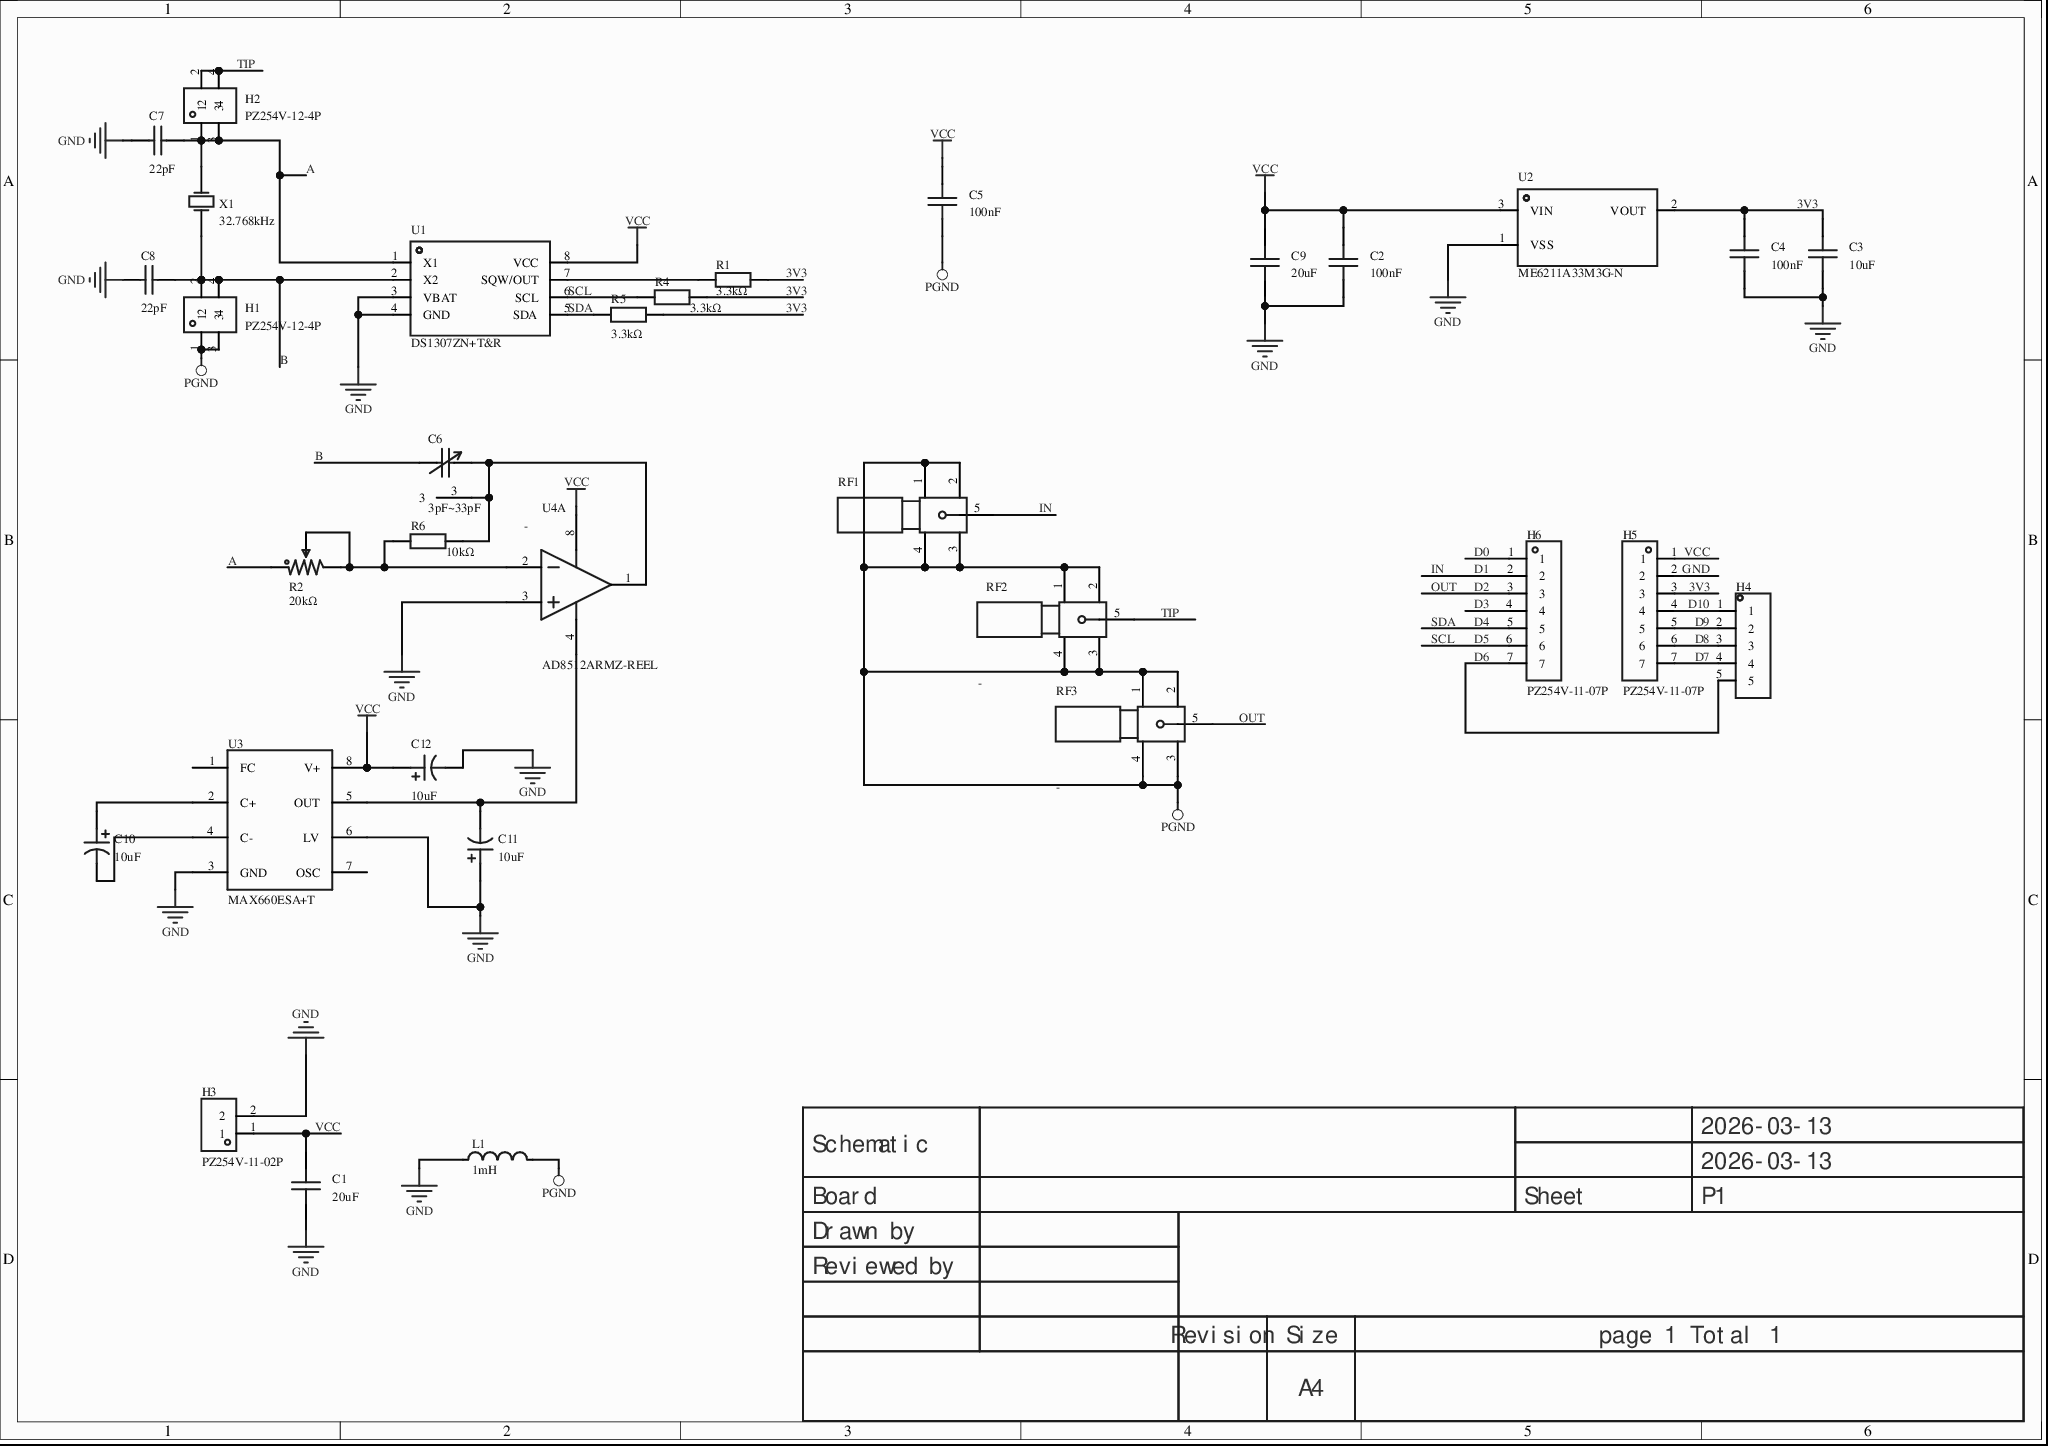
[diagram p0: MISC75269-3.schdoc]
# Altium project MISC75269-2.PrjPcb
1 sheet, 32 parts. Net scope: global (net labels, ports and power ports of the same name join across sheets).
Board file: MISC75269.pcbdoc

## Sheet MISC75269-3.schdoc
size 297 x 209 mm; Version: V1.0; @Project Name: MISC75269; @Update Date: 2026-03-13; @Create Date: 2026-03-13; @Board Name: MISC75269; @Create Time: 17:50:26; @Page Count: 1; @Page No: 1; @Schematic Name: MISC75269; @Update Time: 17:50:26; Size: A4

### Parts
C1  20uF  [CAP-SMD_L1.8-W1.0]
C2  100nF  [C0603]
C3  10uF  [C0603]
C4  100nF  [C0603]
C5  100nF  [C0603]
C6  3pF~33pF  [CAP-ADJ-TH_3P-BD7.6_BFC280811339]
C7  22pF  [C0603]
C8  22pF  [C0603]
C9  20uF  [CAP-SMD_L1.8-W1.0]
C10  10uF  [CAP-SMD_BD5.0-L5.3-W5.3-LS6.0-FD]
C11  10uF  [CAP-SMD_BD5.0-L5.3-W5.3-LS6.0-FD]
C12  10uF  [CAP-SMD_BD5.0-L5.3-W5.3-LS6.0-FD]
H1  PZ254V-12-4P  [HDR-TH_4P-P2.54-V-M-R2-C2-S2.54]
H2  PZ254V-12-4P  [HDR-TH_4P-P2.54-V-M-R2-C2-S2.54]
H3  PZ254V-11-02P  [HDR-TH_2P-P2.54-V-M]
H4  (no value)  [HDR-TH_5P-P2.54-V-M]
H5  PZ254V-11-07P  [HDR-TH_7P-P2.54-V-M]
H6  PZ254V-11-07P  [HDR-TH_7P-P2.54-V-M]
L1  1mH  [IND-TH_BD8.5-P5.00-D0.6]
R1  3.3kΩ  [R0603]
R2  20kΩ  [RES-ADJ-TH_3362P]
R4  3.3kΩ  [R0603]
R5  3.3kΩ  [R0603]
R6  10kΩ  [R0603]
RF1  -  [SMA-TH_KH-SMA-KE-Z]
RF2  -  [SMA-TH_KH-SMA-KE-Z]
RF3  -  [SMA-TH_KH-SMA-KE-Z]
U1  DS1307ZN+T&R  [SOP-8_L4.9-W3.9-P1.27-LS6.0-BL]
U2  ME6211A33M3G-N  [SOT-23-3_L2.9-W1.6-P1.90-LS2.8-BR]
U3  MAX660ESA+T  [SOIC-8_L5.0-W4.0-P1.27-LS6.0-BL]
U4  AD8512ARMZ-REEL  [MSOP-8_L3.0-W3.0-P0.65-LS5.0-TL]  (part A of 2)
X1  32.768kHz  [OSC-TH_BD3.1-P0.8-D0.3]

### Nets
GND: C1.1 C2.1 C3.1 C4.1 C7.2 C8.2 C9.1 C11.1 C12.2 H3.2 H5.2 L1.1 U1.3(VBAT) U1.4(GND) U2.1(VSS) U3.3(GND) U3.6(LV) U4.3(+IN_A)
PGND: C5.1 H1.1 H1.3 L1.2 RF1.1 RF1.2 RF1.3 RF1.4 RF2.1 RF2.2 RF2.3 RF2.4 RF3.1 RF3.2 RF3.3 RF3.4
VCC: C1.2 C2.2 C5.2 C9.2 C12.1 H3.1 H5.1 U1.8(VCC) U2.3(VIN) U3.8(V+) U4.8(V+)
3V3: C3.2 C4.2 H5.3 R1.2 R4.1 R5.1 U2.2(VOUT)
A: C7.1 H2.1 H2.3 R2.1 U1.1(X1) X1.2(OSC2)
B: C6.1 C8.1 H1.2 H1.4 U1.2(X2) X1.1(OSC1)
D0: H6.1
D1: H6.2 RF1.5  [also labelled IN]
D2: H6.3 RF3.5  [also labelled OUT]
D3: H6.4
D4: H6.5 R5.2 U1.5(SDA)  [also labelled SDA]
D5: H6.6 R4.2 U1.6(SCL)  [also labelled SCL]
D6: H4.5 H6.7
D7: H4.4 H5.7
D8: H4.3 H5.6
D9: H4.2 H5.5
D10: H4.1 H5.4
TIP: H2.2 H2.4 RF2.5
NetC6_2: C6.2 C6.3 R6.1 U4.1(OUT_A)
NetC10_1: C10.1 U3.2(C+)
NetC10_2: C10.2 U3.4(C-)
NetC11_2: C11.2 U3.5(OUT) U4.4(V-)
NetR1_1: R1.1 U1.7(SQW/OUT)
NetR2_2: R2.2 R2.3 R6.2 U4.2(-IN_A)

Not connected (* = marked no-connect by the designer): U3 1(FC)* 7(OSC)*

### Notes on the sheet
- 2026-03-13
- Schematic
- Board
- Sheet
- P1
- Drawn by
- Reviewed by
- Revision
- Size
- A4
- page 1 Total 1

### Library data of the parts
C1 C9 = GRMJN7R61C206ME05D: Capacitance:20uF;Tolerance:±20%;Rated voltage:16V;Temperature coefficient:X5R;; Manufacturer: muRata(村田); AddInBom: yes; ModelId: 7fafba264af843cd9b63e401151876ee0819f05c4eef4c71ace90d822a990e87; ModelTransform: 70.866,39.37394,0,0,0,0,0,0,0; Tolerance: ±20%; Voltage Rating: 16V; Temperature Coefficient: X5R; Symbol: GRMJN7R61C206ME05D; Device: GRMJN7R61C206ME05D; LCSC Part Name: 20uF ±20% 16V; SupplierPart: C6565591; ManufacturerPart: GRMJN7R61C206ME05D; Supplier Footprint: 0704; JLCPCB Part Class: Extended Part; Datasheet: example.com/datasheet/GRMJN7R61C206ME05D/7519706.html; Supplier: LCSC; ConvertToPcb: yes; FootprintName: CAP-SMD_L1.8-W1.0; ModelName: CAP-SMD_L1.8-W1.0; Value: 20uF
C2 C4 C5 = CGA0603X7R104K500JT: Capacitance:100nF;Tolerance:±10%;Rated voltage:50V;Temperature coefficient:X7R;; Manufacturer: HRE(芯声); AddInBom: yes; ModelId: ac125912035d415993ca9572d50418b10819f05c4eef4c71ace90d822a990e87; ModelName: C0603_L1.6-W0.8-H0.8; ModelTransform: 62.992,31.496,0,0,0,0,0,0,0; Tolerance: ±10%; Voltage Rating: 50V; Temperature Coefficient: X7R; Symbol: CGA0603X7R104K500JT; Device: CGA0603X7R104K500JT; LCSC Part Name: 100nF ±10% 50V; SupplierPart: C6119867; ManufacturerPart: CGA0603X7R104K500JT; Supplier Footprint: 0603; JLCPCB Part Class: Extended Part; Datasheet: example.com/datasheet/CGA0603X7R104K500JT/7062573.html; Supplier: LCSC; ConvertToPcb: yes; FootprintName: C0603; Value: 100nF
C3 = CGA0603X5R106K100JT: Capacitance:10uF;Tolerance:±10%;Rated voltage:10V;Temperature coefficient:X5R;; Manufacturer: HRE(芯声); AddInBom: yes; ModelId: ac125912035d415993ca9572d50418b10819f05c4eef4c71ace90d822a990e87; ModelName: C0603_L1.6-W0.8-H0.8; ModelTransform: 62.992,31.496,0,0,0,0,0,0,0; Tolerance: ±10%; Voltage Rating: 10V; Temperature Coefficient: X5R; Symbol: CGA0603X5R106K100JT; Device: CGA0603X5R106K100JT; LCSC Part Name: 10uF ±10% 10V; SupplierPart: C6119842; ManufacturerPart: CGA0603X5R106K100JT; Supplier Footprint: 0603; JLCPCB Part Class: Extended Part; Datasheet: example.com/datasheet/CGA0603X5R106K100JT/7062548.html; Supplier: LCSC; ConvertToPcb: yes; FootprintName: C0603; Value: 10uF
C6 = BFC280811339: Capacitance:3pF~33pF;Rated voltage:250V;Charge:-;; Manufacturer: VISHAY(威世); AddInBom: yes; ModelId: cf28104b1ba149229588c665311718d80819f05c4eef4c71ace90d822a990e87; ModelTransform: 334.645,298.957,0,0,0,0,-15.748,0,-157.48; Voltage Rating: 250V; Symbol: BFC280811339; Device: BFC280811339; LCSC Part Name: 3pF~33pF 250V; SupplierPart: C3273212; ManufacturerPart: BFC280811339; Supplier Footprint: 插件; JLCPCB Part Class: Extended Part; Datasheet: example.com/datasheet/BFC280811339/3836109.html; Supplier: LCSC; ConvertToPcb: yes; FootprintName: CAP-ADJ-TH_3P-BD7.6_BFC280811339; ModelName: CAP-ADJ-TH_3P-BD7.6_BFC280811339; Value: 3pF~33pF; Q @ Frequency: -; Operating Temperature: -40℃~+70℃; Height - Seated(Max): 10mm
C7 C8 = CL10C220JB8NNNC: Capacitance:22pF;Tolerance:±5%;Rated voltage:50V;Temperature coefficient:C0G;; Manufacturer: SAMSUNG(三星); AddInBom: yes; ModelId: ac125912035d415993ca9572d50418b10819f05c4eef4c71ace90d822a990e87; ModelName: C0603_L1.6-W0.8-H0.8; ModelTransform: 62.992,31.496,0,0,0,0,0,0,0; Tolerance: ±5%; Voltage Rating: 50V; Temperature Coefficient: C0G; Symbol: CL10C220JB8NNNC; Device: CL10C220JB8NNNC; LCSC Part Name: 22pF ±5% 50V; SupplierPart: C1653; ManufacturerPart: CL10C220JB8NNNC; Supplier Footprint: 0603; JLCPCB Part Class: Basic Part; Datasheet: example.com/datasheet/CL10C220JB8NNNC/2005.html; Supplier: LCSC; ConvertToPcb: yes; FootprintName: C0603; Value: 22pF
C10-C12 = JVJ50v10M5x5: Capacitance:10uF;Tolerance:±20%;Rated voltage:50V;Ripple current:18mA@120Hz;; Manufacturer: JIERR(捷而瑞); 3D Model: ed942b427de741e3aabba01c64b2d7230819f05c4eef4c71ace90d822a990e87; 3D Model Transform: 236.22,208.661,0,0,0,0,-0.001,-0.003,0; Tolerance: ±20%; Voltage Rating: 50V; Lifetime: 2000hrs@105℃; AddInBom: yes; Symbol: JVJ50V10M5X5; Device: JVJ50v10M5x5; LCSC Part Name: 10uF ±20% 50V; Supplier Part: C46550416; Manufacturer Part: JVJ50v10M5x5; Supplier Footprint: SMD,D5xL5.4mm; JLCPCB Part Class: Extended Part; Datasheet: example.com/datasheet/JVJ50v10M5x5/48680110.html; Supplier: LCSC; Value: 10uF; Ripple Current: 18mA@120Hz; Diameter: 5mm; Height - Seated (Max): 5.4mm; Operating Temperature: -55℃~+105℃; ConvertToPcb: yes; FootprintName: CAP-SMD_BD5.0-L5.3-W5.3-LS6.0-FD; ModelName: CAP-SMD_BD5.0-L5.3-W5.3-LS6.0-FD
H1 H2 = PZ254V-12-4P: Pin structure:2x2P;Pitch:2.54mm;Row spacing:2.54mm;Round/square pin:Square pin;Mounting:Through-hole;Rows:Double row;Total pins:4P;Rated current:-;Rated voltage:-;Mating pin length:6mm;Plastic height:2.5mm;Tail length:3mm;Contact material:Brass;Contact plating:-;Operating temperature:-40℃~+105℃;Color:Black;; Manufacturer: XFCN(兴飞); AddInBom: yes; ModelId: 396726ecc332483f84428c142640bc150819f05c4eef4c71ace90d822a990e87; ModelName: HDR-TH_4P-P2.54-M-LI-2X2P; ModelTransform: 200,200,0,0,0,0,0,0,-118.11; Pin Structure: 2x2P; Pitch: 2.54mm; Circluar Pins/Square Pins: Square; Symbol: PZ254V-12-4P; Device: PZ254V-12-4P; LCSC Part Name: 2x2P 间距:2.54mm 方针 直插; SupplierPart: C492419; ManufacturerPart: PZ254V-12-4P; Supplier Footprint: 插件,P=2.54mm; JLCPCB Part Class: Extended Part; Datasheet: example.com/datasheet/PZ254V-12-4P/502975.html; Supplier: LCSC; ConvertToPcb: yes; FootprintName: HDR-TH_4P-P2.54-V-M-R2-C2-S2.54; Row Spacing: 2.54mm; Mounting Type: Through-hole; Number of Rows: Double row; Number of Pins: 4P; Current Rating: -; Voltage Rating (Max): -; Length of Mating Pin: 6mm; Insulation Height: 2.5mm; Length of End Connection Pin: 3mm; Contact Material: Brass; Contact Plating: -; Operating Temperature: -40℃~+105℃; Color: Black
H3 = PZ254V-11-02P: Pin structure:1x2P;Pitch:2.54mm;Row spacing:-;Round/square pin:Square pin;Mounting:Through-hole;Rows:Single row;Total pins:2P;Rated current:-;Rated voltage:-;Mating pin length:6mm;Plastic height:2.5mm;Tail length:3mm;Contact material:Brass;Contact plating:-;Operating temperature:-40℃~+105℃;Color:Black;; Manufacturer: XFCN(兴飞); AddInBom: yes; ModelId: e35305ec3aa84b66b849f914b715e73f0819f05c4eef4c71ace90d822a990e87; ModelName: HDR2.54-M-LI-1X2P; ModelTransform: 200,100,0,0,0,0,0,0,-118.11; Pin Structure: 1x2P; Pitch: 2.54mm; Circluar Pins/Square Pins: Square; Symbol: PZ254V-11-02P; Device: PZ254V-11-02P; LCSC Part Name: 1x2P 间距:2.54mm 方针 直插; SupplierPart: C492401; ManufacturerPart: PZ254V-11-02P; Supplier Footprint: 插件,P=2.54mm; JLCPCB Part Class: Extended Part; Datasheet: example.com/datasheet/PZ254V-11-02P/502957.html; Supplier: LCSC; ConvertToPcb: yes; FootprintName: HDR-TH_2P-P2.54-V-M; Row Spacing: -; Mounting Type: Through-hole; Number of Rows: Single row; Number of Pins: 2P; Current Rating: -; Voltage Rating (Max): -; Length of Mating Pin: 6mm; Insulation Height: 2.5mm; Length of End Connection Pin: 3mm; Contact Material: Brass; Contact Plating: -; Operating Temperature: -40℃~+105℃; Color: Black
H4 = HDR-M_2.54_1x5P: Symbol: MTP125-1105S1; ConvertToPcb: yes; ModelId: 47d466e4a34f4fc5bc626cf773a24dd50819f05c4eef4c71ace90d822a990e87; ModelName: HDR-TH_5P-P2.54-M-LI-1X5P; ModelTransform: 499.999,100,0,0,0,0,0,0,-118.11; Device: HDR-M_2.54_1x5P; AddInBom: yes; SupplierPart: C358687; Supplier Footprint: 插件; FootprintName: HDR-TH_5P-P2.54-V-M
H5 H6 = PZ254V-11-07P: Pin structure:1x7P;Pitch:2.54mm;Row spacing:-;Round/square pin:Square pin;Mounting:Through-hole;Rows:Single row;Total pins:7P;Rated current:-;Rated voltage:-;Mating pin length:6mm;Plastic height:2.5mm;Tail length:3mm;Contact material:Brass;Contact plating:-;Operating temperature:-40℃~+105℃;Color:Black;; Manufacturer: XFCN(兴飞); AddInBom: yes; ModelId: 3f496cdc752348c6a5e9157bbaceaf960819f05c4eef4c71ace90d822a990e87; ModelName: HDR-TH_7P-P2.54-M-LI-1X7P; ModelTransform: 690.1561,98.425,0,0,0,0,0,0,-118.11; Pin Structure: 1x7P; Pitch: 2.54mm; Circluar Pins/Square Pins: Square; Symbol: PZ254V-11-07P; Device: PZ254V-11-07P; LCSC Part Name: 1x7P 间距:2.54mm 方针 直插; SupplierPart: C492406; ManufacturerPart: PZ254V-11-07P; Supplier Footprint: 插件,P=2.54mm; JLCPCB Part Class: Extended Part; Datasheet: example.com/upload/public/pdf/source/20200309/C492406_654C533EE691117E22DD9F76C114C2D9.pdf; Supplier: LCSC; ConvertToPcb: yes; FootprintName: HDR-TH_7P-P2.54-V-M; Row Spacing: -; Mounting Type: Through-hole; Number of Rows: Single row; Number of Pins: 7P; Current Rating: -; Voltage Rating (Max): -; Length of Mating Pin: 6mm; Insulation Height: 2.5mm; Length of End Connection Pin: 3mm; Contact Material: Brass; Contact Plating: -; Operating Temperature: -40℃~+105℃; Color: Black
L1 = SLP0810R-102MTT: Inductance:1mH;Tolerance:±20%;Rated current:500mA;Type:I-shaped inductor;; Manufacturer: Sunltech(顺磁); AddInBom: yes; ModelId: f824c3cd5f0947e0ad34b4cb921321ba0819f05c4eef4c71ace90d822a990e87; ModelName: IND-TH_BD8.5-H8.3-P5.00-D0.6; ModelTransform: 334.645,334.645,0,0,0,0,-0.005,0,-196.85; Tolerance: ±20%; Current Rating: 500mA; DC Resistance(DCR): 1.8Ω; Symbol: SLP0810R-102MTT; Device: SLP0810R-102MTT; LCSC Part Name: 1mH ±20%; SupplierPart: C364093; ManufacturerPart: SLP0810R-102MTT; Supplier Footprint: 插件,D8.5xL12mm; JLCPCB Part Class: Extended Part; Datasheet: example.com/datasheet/SLP0810R-102MTT/338381.html; Supplier: LCSC; ConvertToPcb: yes; FootprintName: IND-TH_BD8.5-P5.00-D0.6; Value: 1mH; Type: I-shaped inductor
R1 R4 R5 = 0603WAF3301T5E: Resistor type:Thick film resistor;Resistance:3.3kΩ;Tolerance:±1%;Power:100mW;Working voltage:75V;Temperature coefficient:±100ppm/℃;; Manufacturer: UNI-ROYAL(厚声); AddInBom: yes; ModelId: fc143cca1e79419f9cd78b61e9279f080819f05c4eef4c71ace90d822a990e87; ModelTransform: 31.8897,63.7794,0,90,0,0,0,0,0; Tolerance: ±1%; Power(Watts): 100mW; Voltage-Supply(Max): 75V; Symbol: 0603WAF3301T5E; Device: 0603WAF3301T5E; LCSC Part Name: 3.3kΩ ±1% 100mW 厚膜电阻; SupplierPart: C22978; ManufacturerPart: 0603WAF3301T5E; Supplier Footprint: 0603; JLCPCB Part Class: Basic Part; Datasheet: example.com/datasheet/0603WAF3301T5E/23705.html; Supplier: LCSC; ConvertToPcb: yes; FootprintName: R0603; ModelName: R0603; Type: Thick film resistor; Value: 3.3kΩ; Temperature Coefficient: ±100ppm/℃; Operating Temperature: -55℃~+155℃
R2 = 3362P-1-103_C48997914: Resistance:10kΩ;Tolerance:±10%;Power:500mW;Temperature coefficient:±250ppm/℃;; Manufacturer: JIERR(捷而瑞); AddInBom: yes; ModelId: b1c5cb968ae748a39271ba681de641230819f05c4eef4c71ace90d822a990e87; ModelName: 3362P; ModelTransform: 271.653,279.527,0,0,0,0,0,-49.803,-232.283; Tolerance: ±10%; Power(Watts): 500mW; Number of Turns: 1; Symbol: 3362P-1-103_C48997914; Device: 3362P-1-103_C48997914; Value: 20kΩ; LCSC Part Name: 玻璃釉预调电位器; ManufacturerPart: 3362P-1-103; Supplier Footprint: 插件-3P,7x6.8mm; JLCPCB Part Class: Extended Part; Datasheet: example.com/datasheet/3362P-1-103/51342050.html; Supplier: LCSC; ConvertToPcb: yes; FootprintName: RES-ADJ-TH_3362P; Temperature Coefficient: ±250ppm/℃
R6 = 0603WAF3301T5E: Resistor type:Thick film resistor;Resistance:3.3kΩ;Tolerance:±1%;Power:100mW;Working voltage:75V;Temperature coefficient:±100ppm/℃;; Manufacturer: UNI-ROYAL(厚声); 3D Model: fc143cca1e79419f9cd78b61e9279f080819f05c4eef4c71ace90d822a990e87; 3D Model Transform: 31.8897,63.7794,0,90,0,0,0,0,0; Tolerance: ±1%; Power(Watts): 100mW; Voltage-Supply(Max): 75V; AddInBom: yes; Symbol: 0603WAF3301T5E; Device: 0603WAF3301T5E; LCSC Part Name: 3.3kΩ ±1% 100mW 厚膜电阻; Manufacturer Part: 0603WAF3301T5E; Supplier Footprint: 0603; JLCPCB Part Class: Basic Part; Datasheet: example.com/datasheet/0603WAF3301T5E/23705.html; Supplier: LCSC; Type: Thick film resistor; Value: 10kΩ; Temperature Coefficient: ±100ppm/℃; Operating Temperature: -55℃~+155℃; ConvertToPcb: yes; FootprintName: R0603; ModelName: R0603
RF1-RF3 = KH-SMA-KE-Z: Connector type:Board mount;Interface type:Jack;Port count:1;Interface diameter:6.2mm;Interface length/height:8mm;Frequency:-;RF series:SMA;Impedance:-;Style:Straight pin;Operating temperature:-;; Manufacturer: kinghelm(金航标); AddInBom: yes; ModelId: 4ccb1f0943094bfb8432c24484a7ccf00819f05c4eef4c71ace90d822a990e87; ModelName: ANT-TH_L6.5-W6.5-H13.5-P5.08; ModelTransform: 255.905,255.905,0,0,0,0,-0.005,0.005,-157.48; Interface: Jack; Number of Ports: 1; Interface Diameter: 6.2mm; Interface Length/Height: 8mm; RF Series: SMA; Symbol: KH-SMA-KE-Z; Device: KH-SMA-KE-Z; LCSC Part Name: SMA 内孔 正脚; SupplierPart: C504007; ManufacturerPart: KH-SMA-KE-Z; Supplier Footprint: 插件; JLCPCB Part Class: Extended Part; Datasheet: example.com/datasheet/KH-SMA-KE-Z/516666.html; Supplier: LCSC; ConvertToPcb: yes; FootprintName: SMA-TH_KH-SMA-KE-Z; Connector Type: Board mount; Value: -; Impedance: -; Style: Straight pin; Operating Temperature Range: -
U1 = DS1307ZN+T&R: Interface type:I2C;; Manufacturer: ADI(亚德诺)/MAXIM(美信); AddInBom: yes; ModelId: 75c24a7891ee4dd6bdac16a7163ff87e0819f05c4eef4c71ace90d822a990e87; ModelName: SOP-8_L4.9-W3.9-P1.27-LS6.0-BL-1; ModelTransform: 192.913,236.22,0,0,0,0,0,0,0; Interface: I2C; Voltage - Supply: 4.5V~5.5V; Symbol: DS1307ZN+; Device: DS1307ZN+T&R; LCSC Part Name: 64 x 8，串行，I2C 实时时钟; SupplierPart: C26858; ManufacturerPart: DS1307ZN+T&R; Supplier Footprint: SOP-8; JLCPCB Part Class: Extended Part; Datasheet: example.com/datasheet/DS1307ZN%252BT%2526R/27606.html; Supplier: LCSC; ConvertToPcb: yes; FootprintName: SOP-8_L4.9-W3.9-P1.27-LS6.0-BL; Operating Temperature: -40℃~+85℃
U2 = ME6211A33M3G-N: Output type:Fixed;Working voltage:6V;Output voltage:3.3V;Output current:500mA;Power supply rejection ratio (PSRR):70dB@(1kHz);Output polarity:Positive;; Manufacturer: MICRONE(南京微盟); AddInBom: yes; ModelId: 89cb27a44ab2466697082bb9fd73a7d00819f05c4eef4c71ace90d822a990e87; ModelName: SOT-23-3L_L2.9-W1.6-H1.1-LS2.8-P0.95; ModelTransform: 114.173,110.236,0,90,0,0,0,0,0; Output Type: Fixed; Voltage - Supply: 6V; Output Voltage: 3.3V; Output Current: 500mA; Voltage Dropout: 120mV@(100mA); standby current: 60uA; Noise: 50uVrms; Number of Outputs: 1; Symbol: ME6211A33M3G-N; Device: ME6211A33M3G-N; LCSC Part Name: 输入6V 输出3.3V 500mA; SupplierPart: C168807; ManufacturerPart: ME6211A33M3G-N; Supplier Footprint: SOT-23-3; JLCPCB Part Class: Extended Part; Datasheet: example.com/datasheet/ME6211A33M3G-N/180190.html; Supplier: LCSC; ConvertToPcb: yes; FootprintName: SOT-23-3_L2.9-W1.6-P1.90-LS2.8-BR; Power Supply Rejection Ratio (PSRR): 70dB@(1kHz); Features: Overcurrent protection; enable; short-circuit protection; Operating Temperature: -40℃~+150℃; Output Configuration: Positive
U3 = MAX660ESA+T: CMOS single-chip voltage converter; converts input voltage by inversion or doubling; Manufacturer: ADI(亚德诺)/MAXIM(美信); AddInBom: yes; ModelId: 7abc64c95a1a4a04a4ef38f9097c870b0819f05c4eef4c71ace90d822a990e87; ModelTransform: 192.913,236.22,0,0,0,0,0,0,0; Operating Voltage: 1.5V~5.5V; Quiescent Current: 500uA; Output Resistance: 6.5Ω; Energy Efficiency: 88%; Switching Frequency: 5kHz; Function: Buck-boost; inverting; Output Voltage: -5.5V~-1.5V; 9.35V; Output Current: 100mA; Symbol: MAX660ESA; Device: MAX660ESA+T; LCSC Part Name: CMOS 单芯片电压转换器; SupplierPart: C9957; ManufacturerPart: MAX660ESA+T; Supplier Footprint: SOIC-8; JLCPCB Part Class: Extended Part; Datasheet: example.com/datasheet/MAX660ESA%252BT/10492.html; Supplier: LCSC; ConvertToPcb: yes; FootprintName: SOIC-8_L5.0-W4.0-P1.27-LS6.0-BL; ModelName: SOIC-8_L5.0-W4.0-P1.27-LS6.0-BL; Operating Temperature: -40℃~+85℃
U4 = AD8512ARMZ-REEL: Amplifier count:Dual;Gain bandwidth product (GBP):8MHz;Input bias current (Ib):25pA;Input offset voltage (Vos):80uV;Slew rate (SR):20V/us;Rail-to-rail:-;; Manufacturer: ADI(亚德诺); Relevance: []; AddInBom: yes; ModelId: bedc0aeebe0a475e87aaac88bd02a14b0819f05c4eef4c71ace90d822a990e87; ModelName: MSOP-8_L3.0-W3.0-H1.1-LS4.9-P0.65; ModelTransform: 118.11,192.913,0,270,0,0,0,0,0; Number of Channels: Dual; Gain Bandwidth Product: 8MHz; Ib - Input Bias Current: 25pA; Vos - Input Offset Voltage: 80uV; Common Mode Rejection Ratio(CMRR): 86dB; Slew Rate: 20V/us; Quiescent Current(Iq): 2.2mA; Input Offset Voltage Drift(Vos TC): 1uV/℃; Output Current: 54mA; Dual Supply: -15V~-1.5V; 1.5V~15V; Maximum Power Supply Range (Vdd-Vss): 30V; Noise density(eN): 8nV/√Hz@1kHz; Symbol: AD8512ARMZ-REEL; Device: AD8512ARMZ-REEL; LCSC Part Name: 精确、超低噪声、低输入偏置电流、宽频带JFET运算放大器; SupplierPart: C36723; ManufacturerPart: AD8512ARMZ-REEL; Supplier Footprint: MSOP-8; JLCPCB Part Class: Extended Part; Datasheet: example.com/datasheet/AD8512ARMZ-REEL/37701.html; Supplier: LCSC; ConvertToPcb: yes; FootprintName: MSOP-8_L3.0-W3.0-P0.65-LS5.0-TL; Rail To Rail: -; Operating Temperature: -40℃~+125℃
X1 = X308032768KGB2SC: Crystal type:Through-hole crystal;Frequency:32.768kHz;Frequency deviation at room temperature:±10ppm;Load capacitance:12.5pF;Frequency stability:±20ppm;; Manufacturer: YXC(扬兴晶振); Add into BOM: yes; 3D Model: 67724a3a0ade4f5eaf21dfa08b7e82c8; 3D Model Transform: 399.9992,118.11,0,0,0,0,-196.85,0,-137.795; Normal temperature Frequency Tolerance: ±10ppm; Load Capacitance: 12.5pF; Frequency Stability: ±20ppm; ModelName: OSC-TH_D3.0-W8.0-P0.8; Symbol: X308032768KGB2SC; Device: X308032768KGB2SC; Convert to PCB: yes; LCSC Part Name: YT-38 32.768KHZ 2P 3080 12.5PF ±10PPM -20~70℃; Supplier Part: C52082; Manufacturer Part: X308032768KGB2SC; Supplier Footprint: DT-38; JLCPCB Part Class: Extended Part; Datasheet: example.com/datasheet/X308032768KGB2SC/53096.html; Supplier: LCSC; Type: Through-hole crystal; Value: 32.768kHz; Operating Temperature: -20℃~+70℃; FootprintName: OSC-TH_BD3.1-P0.8-D0.3